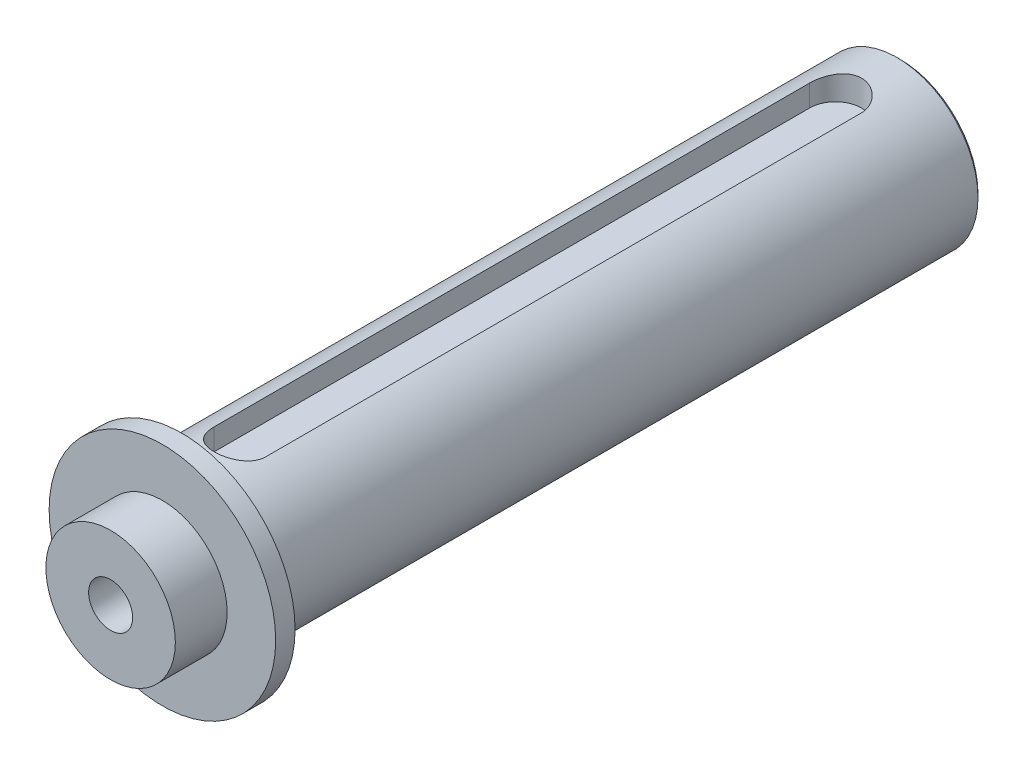
SolidWorks part; units mm, degrees
material "1023 碳钢板 (SS)"
ref_plane "前视基准面" through (0, 0, 0) normal (0, 0, 1) x (1, 0, 0)
ref_plane "上视基准面" through (0, 0, 0) normal (0, 1, 0) x (1, 0, 0)
ref_plane "右视基准面" through (0, 0, 0) normal (1, 0, 0) x (0, 0, -1)
sketch "草图1" plane through (0, 0, 0) normal (0, 0, 1) x (1, 0, 0)
  circle A0 centre (0, 0) radius 12.5
  dimension "D1" = 25
extrude "凸台-拉伸1" add sketch "草图1" along normal blind 111
sketch "草图2" plane through (0, 0, 111) normal (0, 0, 1) x (1, 0, 0)
  circle A0 centre (0, 0) radius 17.5
  dimension "D1" = 35
extrude "凸台-拉伸2" add sketch "草图2" along normal blind 3
sketch "草图3" plane through (0, 0, 114) normal (0, 0, 1) x (1, 0, 0)
  circle A0 centre (0, 0) radius 10
  dimension "D1" = 20
extrude "凸台-拉伸3" add sketch "草图3" along normal blind 8
ref_plane "基准面1" through (0, 12.5, 0) normal (0, 1, 0) x (1, 0, 0)
sketch "草图4" plane through (0, 12.5, 0) normal (0, 1, 0) x (1, 0, 0)
  line L0 (0, -10) -> (0, -102) construction
  line L1 (4, -10) -> (4, -102)
  line L2 (-4, -10) -> (-4, -102)
  line L3 (12.5, 0) -> (-12.5, 0) construction
  arc A0 (4, -10) -> (-4, -10) centre (0, -10) ccw
  arc A1 (-4, -102) -> (4, -102) centre (0, -102) ccw
  point P3 (0, -56)
  dimension "D1" = 4
  dimension "D3" = 10
  dimension "D2" = 92
extrude "切除-拉伸1" cut sketch "草图4" against normal blind 4
hole_wizard "M8 螺纹孔1" positions "草图5" profile "草图6" tap size "M8" standard "GB"
sketch "草图5" plane through (0, 0, 122) normal (0, 0, 1) x (1, 0, 0)
  point P0 (0, 0)
sketch "草图6" plane through (0, 0, 122) normal (1, 0, 0) x (0, -1, 0)
  line L0 (0, 0) -> (0, 25.7929)
  line L1 (0, 25.7929) -> (3.4, 23.75)
  line L2 (3.4, 23.75) -> (3.4, 0)
  line L5 (3.4, 0) -> (0, 0)
  line L10 (0, 25.7929) -> (-3.4, 23.75) construction
  line L11 (0, -6.35) -> (0, 107.95) construction
  dimension "螺纹孔钻头直径" = 6.8
  dimension "螺纹孔钻头深度" = 23.75
  dimension "导头角度" = 118
cosmetic thread "孔螺蚊线1"
hole_wizard "M12 螺纹孔1" positions "草图7" profile "草图8" tap size "M12" standard "GB"
sketch "草图7" plane through (0, 0, 0) normal (0, 0, -1) x (-1, 0, 0)
  point P0 (0, 0)
cosmetic thread "孔螺蚊线2" parameters "D1"=25, "D2"=12
sketch "草图8" plane through (0, 0, 0) normal (1, 0, 0) x (0, 1, 0)
  line L0 (0, 0) -> (0, 33.3144)
  line L1 (0, 33.3144) -> (5.1, 30.25)
  line L2 (5.1, 30.25) -> (5.1, 0)
  line L5 (5.1, 0) -> (0, 0)
  line L10 (0, 33.3144) -> (-5.1, 30.25) construction
  line L11 (0, -6.35) -> (0, 107.95) construction
  dimension "螺纹孔钻头直径" = 10.2
  dimension "螺纹孔钻头深度" = 30.25
  dimension "导头角度" = 118
chamfer "倒角1" distance 0.5 angle 45 1 edges at (12.5, 0, 0)
